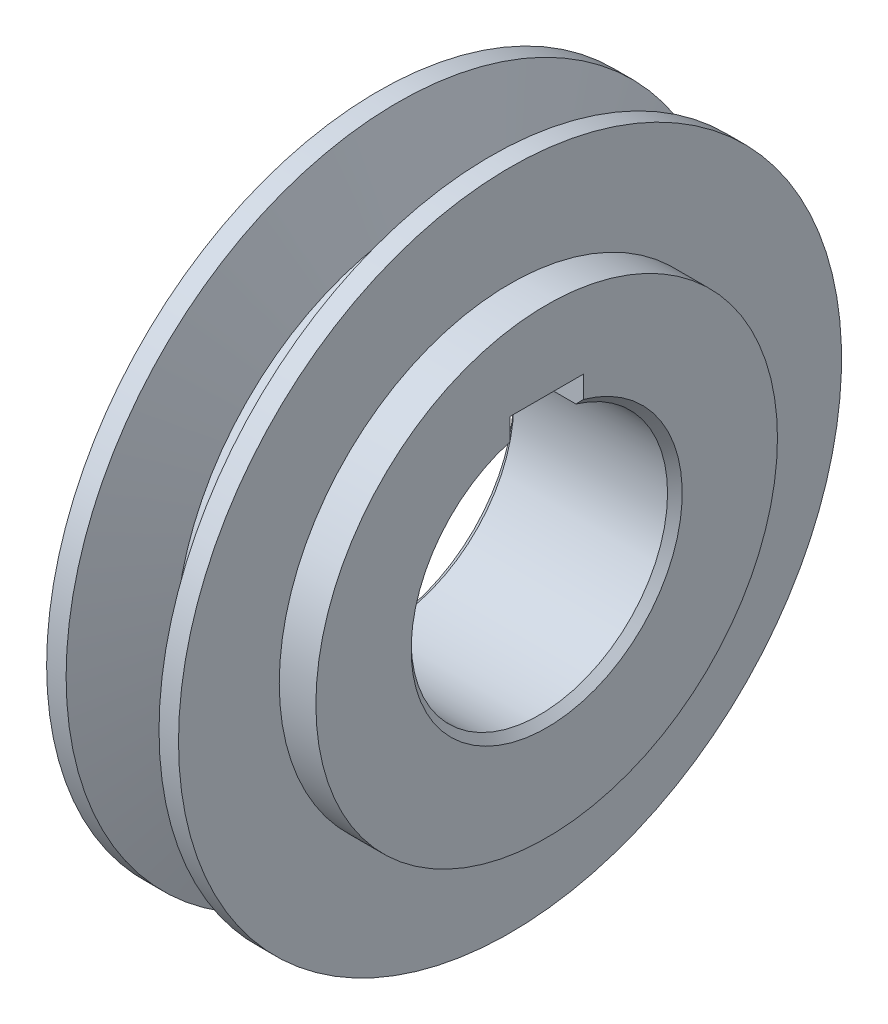
SolidWorks part; units mm, degrees
ref_plane "前视基准面" through (0, 0, 0) normal (0, 0, 1) x (1, 0, 0)
ref_plane "上视基准面" through (0, 0, 0) normal (0, 1, 0) x (1, 0, 0)
ref_plane "右视基准面" through (0, 0, 0) normal (1, 0, 0) x (0, 0, -1)
sketch "草图1" plane through (0, 0, 0) normal (0, 0, 1) x (1, 0, 0)
  line L0 (0, 0) -> (64.8368, 0) construction
  line L1 (0, 17.5) -> (0, 45.25)
  line L2 (0, 45.25) -> (18, 45.25)
  line L3 (18, 45.25) -> (18, 31.5)
  line L4 (18, 31.5) -> (23, 31.5)
  line L5 (23, 31.5) -> (23, 17.5)
  line L6 (23, 17.5) -> (0, 17.5)
  line L7 (2.6592, 45.25) -> (6.1599, 33.8) construction
  line L8 (6.1599, 33.8) -> (11.8401, 33.8) construction
  line L9 (11.8401, 33.8) -> (15.3408, 45.25) construction
  line L10 (0, 42.5) -> (18, 42.5) construction
  line L11 (9, 33.8) -> (9, 17.5) construction
  point P17 (3.5, 42.5)
  point P18 (14.5, 42.5)
  dimension "d2" = 90.5
  dimension "L" = 23
  dimension "B" = 18
  dimension "d" = 35
  dimension "d1" = 63
  dimension "dd" = 85
  dimension "f" = 9
  dimension "槽轮角" = 34
  dimension "bd" = 11
  dimension "hf" = 8.7
  dimension "ha" = 2.75
revolve "旋转1" add sketch "草图1" angle 360 about L0
sketch "草图2" plane through (0, 0, 0) normal (0, 0, 1) x (1, 0, 0)
  line L0 (11.8401, 33.8) -> (15.3408, 45.25) construction
  line L1 (6.1599, 33.8) -> (11.8401, 33.8) construction
  line L2 (2.6592, 45.25) -> (6.1599, 33.8) construction
  line L3 (11.8401, 33.8) -> (15.3408, 45.25)
  line L4 (6.1599, 33.8) -> (11.8401, 33.8)
  line L5 (2.6592, 45.25) -> (6.1599, 33.8)
  line L6 (2.6592, 45.25) -> (15.3408, 45.25)
  line L7 (0, 0) -> (18, 0) construction
  line L8 (18, -31.5) -> (18, 31.5) construction
revolve "切除-旋转1" cut sketch "草图2" angle 360 about L7
chamfer "倒角1" distance 1 2 edges at (23, 0, 17.5) (0, 0, 17.5)
sketch "草图4" plane through (0, 0, 0) normal (-1, 0, 0) x (0, 0, 1)
  line L1 (-5, 16.7705) -> (5, 16.7705)
  line L2 (-5, 16.7705) -> (-5, 20.8)
  line L3 (-5, 20.8) -> (5, 20.8)
  line L4 (5, 16.7705) -> (5, 20.8)
  circle A0 centre (0, 0) radius 17.5 construction
  point P6 (1.7, 20.8)
  dimension "键槽高度" = 20.8
  dimension "键槽宽度" = 10
  dimension "t1" = 3.3
extrude "切除-拉伸1" cut sketch "草图4" against normal through all
